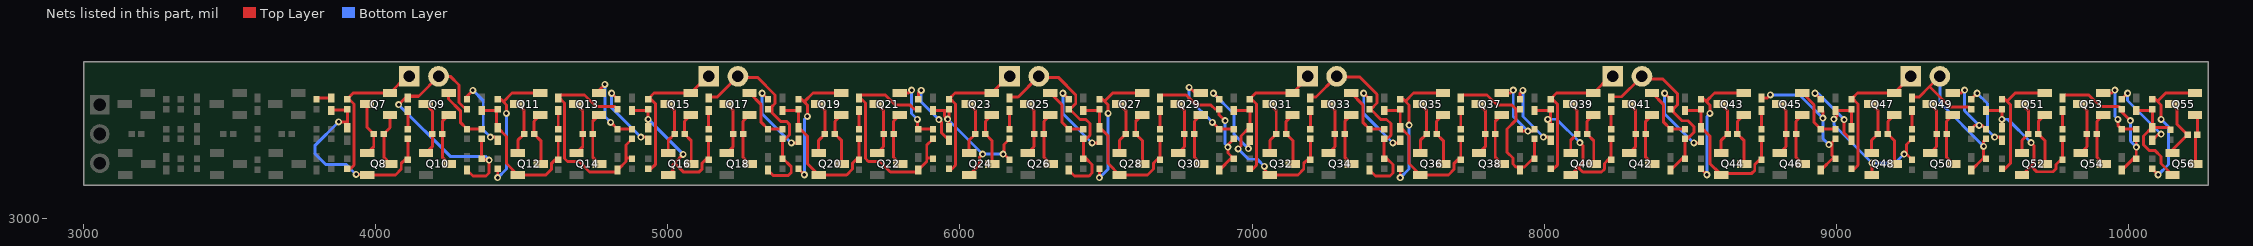
[diagram p0: the nets of this part, all layers, seen from the top]
# Altium PCB MISC51432.pcbdoc (part 2 of 2)
Units mil, origin at the board's own origin, x right, y up, seen from the top; angles counter-clockwise.
Board outline 7274.02 x 423.7 mil, 2 copper layers (Top Layer, Bottom Layer), stack 62.206 mil thick; 257 components, 141 nets, 571 pads, 133 vias.

## Via types
v1: diameter 24.02, hole 12, Top Layer to Bottom Layer, 133 vias

## Nets (pads, with @x,y where several pads share a name; then routed paths per layer and width w, separated by ;. In a path a pad name is that pad's centre, name@x,y a point inside that pad or via, vN(x,y) a via of type N, cw(c..) or ccw(c..) an arc to the next point about the centre after c; other vN are vias at no path point) (continued)
$1N4560: Q7.3 Q8.1 Rb4.2 | length 186.1
  Top Layer w10: Q7.3@3969.94,3391.14 3969.94,3311.66 Rb4.2@3992.96,3288.64 3992.96,3245.18 Q8.1@3971.32,3223.54
$1N4561: Q7.1 Q8.3 Rb4.1 | length 186.3
  Top Layer w10: Rb4.1@4027.04,3288.64 Rb4.1@4027.47,3289.07 ; Q7.1@4048.68,3353.74 4048.68,3310.28 Rb4.1@4027.47,3289.07 ; Q8.3@4050.06,3186.14 4027.47,3208.73 Rb4.1@4027.47,3289.07
$1N4562: C8.2 R6.1 | length 51.8
  Top Layer w10: R6.1@3797.5,3408.18 3801.92,3412.6 C8.2@3847.5,3412.6
$1N4850: C9.1 C10.2 H2.2 R10.2 R11.1 Rs5.2 | length 1018.2
  Top Layer w10: v1(4077.82,3388.97) 4107.82,3418.97 4147.82,3418.97 ; C9.1@4109.62,3412.6 4113.16,3416.14 4145,3416.14 4147.82,3418.97 ; C10.2@4312.5,3164.68 4332.5,3144.68 4377.82,3144.68 4387.82,3154.68 v1(4387.82,3198.97) 4377.82,3198.97 R11.1@4362.5,3214.29 ; R10.2@4312.5,3374.1 4307.04,3374.1 4285,3396.14 4285,3456.14 4255,3486.14 H2.2@4215,3486.14 4147.82,3418.97 ; R11.1@4362.5,3203.18 R11.1@4362.5,3214.29 ; Rs5.2@4362.5,3271.6 R11.1@4362.5,3214.29
  Bottom Layer w10: v1(4077.82,3388.97) 4254.6,3212.19 4374.6,3212.19 v1(4387.82,3198.97)
$1N4855: C9.2 R8.1 | length 64
  Top Layer w10: R8.1@4109.62,3305.68 C9.2@4109.62,3369.68
$1N4859: Q9.3 Q10.1 Rb5.2 | length 186.1
  Top Layer w10: Q9.3@4170.63,3391.14 4193.65,3368.12 Rb5.2@4193.65,3288.64 4193.65,3245.18 Q10.1@4172.01,3223.54
$1N4860: Q9.1 Q10.3 Rb5.1 | length 186.1
  Top Layer w10: Q9.1@4249.37,3353.74 4227.73,3332.1 Rb5.1@4227.73,3288.64 4227.73,3209.16 Q10.3@4250.75,3186.14
$1N4861: Q9.2 Rp5.2 Rs5.1 | length 199
  Top Layer w10: Q9.2@4249.37,3428.54 4249.37,3408.54 4289.37,3368.54 4289.37,3328.81 Rp5.2@4312.5,3305.68 Rs5.1@4362.5,3305.68
$1N5378: Q11.3 Q12.1 Rb6.2 | length 186.1
  Top Layer w10: Q11.3@4484.94,3391.14 4507.96,3368.12 Rb6.2@4507.96,3288.64 4486.32,3267 Q12.1@4486.32,3223.54
$1N5379: Q11.1 Q12.3 Rb6.1 | length 186.1
  Top Layer w10: Q11.1@4563.68,3353.74 4542.04,3332.1 Rb6.1@4542.04,3288.64 4565.06,3265.62 Q12.3@4565.06,3186.14
$1N5380: C12.2 R10.1 | length 252.7
  Top Layer w10: R10.1@4312.5,3408.18 4312.5,3418.18 v1(4332.5,3438.18) ; v1(4392.5,3278.18) 4406.5,3278.18 C12.2@4417.5,3267.18
  Bottom Layer w10: v1(4332.5,3438.18) 4367.86,3402.83 4367.86,3302.83 v1(4392.5,3278.18)
$1N5381: C11.1 C12.1 Q12.2 R12.2 R13.2 Rp6.1 | length 550.3
  Top Layer w10: C11.1@4362.5,3369.68 Rp6.1@4413.08,3369.68 ; Rp6.1@4417.5,3374.1 Rp6.1@4413.08,3369.68 ; R12.2@4624.62,3271.6 R13.2@4624.62,3201.14 4614.62,3201.14 4602.22,3188.74 4602.22,3168.74 4582.22,3148.74 Q12.2@4486.32,3148.74 4447.5,3187.56 4447.5,3280.1 C12.1@4417.5,3310.1 4413.08,3314.52 Rp6.1@4413.08,3369.68
$1N5390: Q11.2 Rp6.2 Rs6.1 | length 468.9
  Top Layer w10: v1(4417.5,3139.1) Rs6.1@4417.5,3169.1 ; Rp6.2@4417.5,3408.18 4427.5,3408.18 4436.89,3398.79 ; v1(4447.5,3359.1) 4447.5,3388.18 4436.89,3398.79 ; Q11.2@4563.68,3428.54 4466.65,3428.54 4436.89,3398.79
  Bottom Layer w10: v1(4417.5,3139.1) 4447.5,3169.1 v1(4447.5,3359.1)
$1N5401: C13.1 C14.2 R14.2 R15.1 Rs7.2 | length 804.1
  Top Layer w10: C13.1@4624.62,3412.6 C13.1@4626.39,3414.37 ; C14.2@4827.5,3164.68 4831.64,3168.82 C14.2@4831.64,3169.62 ; R14.2@4827.5,3374.1 4819,3382.6 4754.62,3382.6 4714.62,3422.6 4634.62,3422.6 C13.1@4626.39,3414.37 ; R15.1@4877.5,3203.18 4873.81,3206.87 4856.39,3206.87 ; Rs7.2@4877.5,3271.6 4856.39,3250.49 4856.39,3206.87 ; C13.1@4626.39,3414.37 4646.39,3394.37 4646.39,3204.37 4656.39,3194.37 4696.39,3194.37 4731.74,3159.01 4821.03,3159.01 C14.2@4831.64,3169.62 ; C14.2@4831.64,3169.62 4856.39,3194.37 4856.39,3206.87
$1N5406: C13.2 R12.1 | length 64
  Top Layer w10: R12.1@4624.62,3305.68 C13.2@4624.62,3369.68
$1N5415: Q13.3 Q14.1 Rb7.2 | length 186.1
  Top Layer w10: Q13.3@4685.63,3391.14 4708.65,3368.12 Rb7.2@4708.65,3288.64 4708.65,3245.18 Q14.1@4687.01,3223.54
$1N5416: Q13.1 Q14.3 Rb7.1 | length 186.1
  Top Layer w10: Q13.1@4764.37,3353.74 4742.73,3332.1 Rb7.1@4742.73,3288.64 4742.73,3209.16 Q14.3@4765.75,3186.14
$1N5417: Q13.2 Rp7.2 Rs7.1 | length 259.1
  Top Layer w10: Q13.2@4764.37,3428.54 4764.37,3438.54 v1(4784.37,3458.54) ; v1(4804.37,3328.54) Rp7.2@4827.5,3305.68 Rs7.1@4877.5,3305.68
  Bottom Layer w10: v1(4784.37,3458.54) 4784.37,3348.54 v1(4804.37,3328.54)
$1N5932: Q15.3 Q16.1 Rb8.2 | length 186.1
  Top Layer w10: Q15.3@4999.94,3391.14 5022.96,3368.12 Rb8.2@5022.96,3288.64 5001.32,3267 Q16.1@5001.32,3223.54
$1N5933: Q15.1 Q16.3 Rb8.1 | length 186.1
  Top Layer w10: Q15.1@5078.68,3353.74 5057.04,3332.1 Rb8.1@5057.04,3288.64 5080.06,3265.62 Q16.3@5080.06,3186.14
$1N5934: C16.2 R14.1 | length 249.3
  Top Layer w10: v1(4807.5,3428.18) R14.1@4827.5,3408.18 ; v1(4907.5,3278.18) 4921.5,3278.18 C16.2@4932.5,3267.18
  Bottom Layer w10: v1(4807.5,3428.18) 4807.5,3378.18 v1(4907.5,3278.18)
$1N5955: C17.1 C18.2 H3.2 R18.2 R19.1 Rs9.2 | length 732.3
  Top Layer w10: C17.1@5139.62,3412.6 5142.45,3415.43 5169.29,3415.43 H3.2@5236.46,3482.61 ; H3.2@5240,3486.14 H3.2@5236.46,3482.61 ; C18.2@5342.5,3164.68 5360.58,3146.6 5412.5,3146.6 5422.5,3156.6 5422.5,3176.6 R19.1@5392.5,3206.6 ; R18.2@5342.5,3374.1 5347.96,3374.1 5355.86,3382 ; R19.1@5392.5,3203.18 R19.1@5392.5,3206.6 ; H3.2@5236.46,3482.61 5306.46,3482.61 5366.46,3422.61 5366.46,3392.61 5355.86,3382 ; 5355.86,3382 5355.86,3362 5385.86,3332 5405.86,3332 5415.86,3322 5415.86,3284.96 5402.5,3271.6 Rs9.2@5392.5,3271.6 R19.1@5392.5,3206.6
$1N5960: C17.2 R16.1 | length 64
  Top Layer w10: R16.1@5139.62,3305.68 C17.2@5139.62,3369.68
$1N5969: Q17.3 Q18.1 Rb9.2 | length 186.1
  Top Layer w10: Q17.3@5200.63,3391.14 5223.65,3368.12 Rb9.2@5223.65,3288.64 5223.65,3245.18 Q18.1@5202.01,3223.54
$1N5970: Q17.1 Q18.3 Rb9.1 | length 186.1
  Top Layer w10: Q17.1@5279.37,3353.74 5257.73,3332.1 Rb9.1@5257.73,3288.64 5257.73,3209.16 Q18.3@5280.75,3186.14
$1N6486: Q19.3 Q20.1 Rb10.2 | length 186.1
  Top Layer w10: Q19.3@5514.94,3391.14 5537.96,3368.12 Rb10.2@5537.96,3288.64 5516.32,3267 Q20.1@5516.32,3223.54
$1N6487: Q19.1 Q20.3 Rb10.1 | length 186.1
  Top Layer w10: Q19.1@5593.68,3353.74 5572.04,3332.1 Rb10.1@5572.04,3288.64 5595.06,3265.62 Q20.3@5595.06,3186.14
$1N6488: C20.2 R18.1 | length 268.4
  Top Layer w10: v1(5322.5,3428.18) R18.1@5342.5,3408.18 ; v1(5422.5,3258.18) 5438.5,3258.18 C20.2@5447.5,3267.18
  Bottom Layer w10: v1(5322.5,3428.18) 5322.5,3358.18 v1(5422.5,3258.18)
$1N6489: C19.1 C20.1 Q20.2 R20.2 R21.2 Rp10.1 | length 554.4
  Top Layer w10: C19.1@5392.5,3369.68 5443.08,3369.68 Rp10.1@5447.5,3374.1 C20.1@5447.5,3311.6 ; C20.1@5447.5,3310.1 C20.1@5447.5,3311.6 ; R20.2@5654.62,3271.6 R21.2@5654.62,3201.14 5644.62,3201.14 5632.22,3188.74 5632.22,3168.74 5612.22,3148.74 Q20.2@5516.32,3148.74 5477.5,3187.56 5477.5,3281.6 C20.1@5447.5,3311.6
$1N6498: Q19.2 Rp10.2 Rs10.1 | length 448.9
  Top Layer w10: Rs10.1@5447.5,3169.1 v1(5467.5,3149.1) ; Rp10.2@5447.5,3408.18 5457.5,3408.18 5466.89,3398.79 ; v1(5477.5,3349.1) 5477.5,3388.18 5466.89,3398.79 ; Q19.2@5593.68,3428.54 5496.65,3428.54 5466.89,3398.79
  Bottom Layer w10: v1(5467.5,3149.1) 5467.5,3339.1 v1(5477.5,3349.1)
$1N6509: C21.1 C22.2 R22.2 R23.1 Rs11.2 | length 797.4
  Top Layer w10: C21.1@5654.62,3412.6 C21.1@5656.39,3414.37 ; R22.2@5857.5,3374.1 5843.12,3374.1 5829.97,3387.25 5779.97,3387.25 5744.62,3422.6 5664.62,3422.6 C21.1@5656.39,3414.37 ; R23.1@5907.5,3203.18 5903.81,3206.87 5886.39,3206.87 ; Rs11.2@5907.5,3271.6 5886.39,3250.49 5886.39,3206.87 ; C21.1@5656.39,3414.37 5676.39,3394.37 5676.39,3204.37 5686.39,3194.37 5726.39,3194.37 5761.74,3159.01 5851.03,3159.01 5886.39,3194.37 5886.39,3206.87
$1N6514: C21.2 R20.1 | length 64
  Top Layer w10: R20.1@5654.62,3305.68 C21.2@5654.62,3369.68
$1N6523: Q21.3 Q22.1 Rb11.2 | length 186.1
  Top Layer w10: Q21.3@5715.63,3391.14 5738.65,3368.12 Rb11.2@5738.65,3288.64 5738.65,3245.18 Q22.1@5717.01,3223.54
$1N6524: Q21.1 Q22.3 Rb11.1 | length 186.1
  Top Layer w10: Q21.1@5794.37,3353.74 5772.73,3332.1 Rb11.1@5772.73,3288.64 5772.73,3209.16 Q22.3@5795.75,3186.14
$1N6525: Q21.2 Rp11.2 Rs11.1 | length 236.6
  Top Layer w10: Q21.2@5794.37,3428.54 5824.37,3428.54 v1(5834.37,3438.54) ; v1(5854.37,3338.54) 5854.37,3308.81 Rp11.2@5857.5,3305.68 Rs11.1@5907.5,3305.68
  Bottom Layer w10: v1(5834.37,3438.54) 5834.37,3358.54 v1(5854.37,3338.54)
$1N7040: Q23.3 Q24.1 Rb12.2 | length 186.1
  Top Layer w10: Q23.3@6029.94,3391.14 6052.96,3368.12 Rb12.2@6052.96,3288.64 6031.32,3267 Q24.1@6031.32,3223.54
$1N7041: Q23.1 Q24.3 Rb12.1 | length 186.1
  Top Layer w10: Q23.1@6108.68,3353.74 6087.04,3332.1 Rb12.1@6087.04,3288.64 6110.06,3265.62 Q24.3@6110.06,3186.14
$1N7042: C24.2 R22.1 | length 244.5
  Top Layer w10: R22.1@5857.5,3408.18 5857.5,3428.18 v1(5867.5,3438.18) ; v1(5927.5,3338.18) 5937.5,3328.18 5937.5,3292.18 C24.2@5962.5,3267.18
  Bottom Layer w10: v1(5867.5,3438.18) 5867.5,3398.18 v1(5927.5,3338.18)
$1N7063: C25.1 C26.2 H4.2 R26.2 R27.1 Rs13.2 | length 734.5
  Top Layer w10: C25.1@6169.62,3412.6 6172.45,3415.43 6199.29,3415.43 H4.2@6266.46,3482.61 ; H4.2@6270,3486.14 H4.2@6266.46,3482.61 ; C26.2@6372.5,3164.68 6392.5,3144.68 6442.5,3144.68 6452.5,3154.68 6452.5,3184.1 6432.5,3204.1 R27.1@6422.5,3204.1 ; R26.2@6372.5,3374.1 R26.2@6375.46,3374.1 ; R27.1@6422.5,3203.18 R27.1@6422.5,3204.1 ; H4.2@6266.46,3482.61 6336.46,3482.61 6396.46,3422.61 6396.46,3392.61 6377.96,3374.1 R26.2@6375.46,3374.1 ; R26.2@6375.46,3374.1 6410.82,3338.75 6430.82,3338.75 6445.46,3324.1 6445.46,3284.56 6432.5,3271.6 Rs13.2@6422.5,3271.6 R27.1@6422.5,3204.1
$1N7068: C25.2 R24.1 | length 64
  Top Layer w10: R24.1@6169.62,3305.68 C25.2@6169.62,3369.68
$1N7077: Q25.3 Q26.1 Rb13.2 | length 186.1
  Top Layer w10: Q25.3@6230.63,3391.14 6253.65,3368.12 Rb13.2@6253.65,3288.64 6253.65,3245.18 Q26.1@6232.01,3223.54
$1N7078: Q25.1 Q26.3 Rb13.1 | length 186.1
  Top Layer w10: Q25.1@6309.37,3353.74 6287.73,3332.1 Rb13.1@6287.73,3288.64 6287.73,3209.16 Q26.3@6310.75,3186.14
$1N7594: Q27.3 Q28.1 Rb14.2 | length 186.1
  Top Layer w10: Q27.3@6544.94,3391.14 6567.96,3368.12 Rb14.2@6567.96,3288.64 6546.32,3267 Q28.1@6546.32,3223.54
$1N7595: Q27.1 Q28.3 Rb14.1 | length 186.1
  Top Layer w10: Q27.1@6623.68,3353.74 6602.04,3332.1 Rb14.1@6602.04,3288.64 6625.06,3265.62 Q28.3@6625.06,3186.14
$1N7596: C28.2 R26.1 | length 268.4
  Top Layer w10: v1(6352.5,3428.18) R26.1@6372.5,3408.18 ; v1(6452.5,3258.18) 6468.5,3258.18 C28.2@6477.5,3267.18
  Bottom Layer w10: v1(6352.5,3428.18) 6352.5,3358.18 v1(6452.5,3258.18)
$1N7597: C27.1 C28.1 Q28.2 R28.2 R29.2 Rp14.1 | length 554.4
  Top Layer w10: C27.1@6422.5,3369.68 6473.08,3369.68 Rp14.1@6477.5,3374.1 C28.1@6477.5,3311.6 ; C28.1@6477.5,3310.1 C28.1@6477.5,3311.6 ; R28.2@6684.62,3271.6 R29.2@6684.62,3201.14 6674.62,3201.14 6662.22,3188.74 6662.22,3168.74 6642.22,3148.74 Q28.2@6546.32,3148.74 6507.5,3187.56 6507.5,3281.6 C28.1@6477.5,3311.6
$1N7606: Q27.2 Rp14.2 Rs14.1 | length 469.9
  Top Layer w10: v1(6477.5,3139.1) Rs14.1@6477.5,3169.1 ; Rp14.2@6477.5,3408.18 6487.5,3408.18 6495.13,3400.55 ; v1(6507.5,3359.1) 6507.5,3388.18 6495.13,3400.55 ; Q27.2@6623.68,3428.54 6523.11,3428.54 6495.13,3400.55
  Bottom Layer w10: v1(6477.5,3139.1) 6507.5,3169.1 v1(6507.5,3359.1)
$1N7617: C29.1 C30.2 R30.2 R31.1 Rs15.2 | length 517
  Top Layer w10: C29.1@6684.62,3412.6 6694.62,3422.6 6774.62,3422.6 6809.97,3387.25 6859.97,3387.25 6873.12,3374.1 R30.2@6887.5,3374.1 6887.5,3354.1 v1(6907.5,3334.1) ; C30.2@6887.5,3164.68 R31.1@6931.64,3208.82 ; R31.1@6937.5,3203.18 6917.5,3223.18 v1(6917.5,3244.1) 6917.5,3251.6 Rs15.2@6937.5,3271.6
  Bottom Layer w10: v1(6907.5,3334.1) 6907.5,3254.1 v1(6917.5,3244.1)
$1N7622: C29.2 R28.1 | length 64
  Top Layer w10: R28.1@6684.62,3305.68 C29.2@6684.62,3369.68
$1N7631: Q29.3 Q30.1 Rb15.2 | length 186.1
  Top Layer w10: Q29.3@6745.63,3391.14 6768.65,3368.12 Rb15.2@6768.65,3288.64 6768.65,3245.18 Q30.1@6747.01,3223.54
$1N7632: Q29.1 Q30.3 Rb15.1 | length 186.1
  Top Layer w10: Q29.1@6824.37,3353.74 6802.73,3332.1 Rb15.1@6802.73,3288.64 6802.73,3209.16 Q30.3@6825.75,3186.14
$1N7633: Q29.2 Rp15.2 Rs15.1 | length 283.9
  Top Layer w10: v1(6784.37,3448.54) 6804.37,3428.54 Q29.2@6824.37,3428.54 ; v1(6864.37,3328.54) Rp15.2@6887.5,3305.68 Rs15.1@6937.5,3305.68
  Bottom Layer w10: v1(6784.37,3448.54) 6784.37,3408.54 v1(6864.37,3328.54)
$1N8148: Q31.3 Q32.1 Rb16.2 | length 186.1
  Top Layer w10: Q31.3@7059.94,3391.14 7082.96,3368.12 Rb16.2@7082.96,3288.64 7061.32,3267 Q32.1@7061.32,3223.54
$1N8149: Q31.1 Q32.3 Rb16.1 | length 186.1
  Top Layer w10: Q31.1@7138.68,3353.74 7117.04,3332.1 Rb16.1@7117.04,3288.64 7140.06,3265.62 Q32.3@7140.06,3186.14
$1N8150: C32.2 R30.1 | length 299.1
  Top Layer w10: v1(6867.5,3428.18) R30.1@6887.5,3408.18 ; v1(6987.5,3238.18) 6987.5,3262.18 C32.2@6992.5,3267.18
  Bottom Layer w10: v1(6867.5,3428.18) 6938.21,3357.47 6938.21,3287.47 v1(6987.5,3238.18)
$1N8171: C33.1 C34.2 H5.2 R34.2 R35.1 Rs17.2 | length 737
  Top Layer w10: C33.1@7199.62,3412.6 7202.45,3415.43 7219.29,3415.43 H5.2@7288.23,3484.37 ; H5.2@7290,3486.14 H5.2@7288.23,3484.37 ; C34.2@7402.5,3164.68 7422.5,3144.68 7472.5,3144.68 7482.5,3154.68 7482.5,3184.1 7462.5,3204.1 R35.1@7452.5,3204.1 ; R34.2@7402.5,3374.1 R34.2@7405.46,3374.1 ; R35.1@7452.5,3203.18 R35.1@7452.5,3204.1 ; H5.2@7288.23,3484.37 7368.23,3484.37 7428.23,3424.37 7428.23,3394.37 7407.96,3374.1 R34.2@7405.46,3374.1 ; R34.2@7405.46,3374.1 7440.82,3338.75 7460.82,3338.75 7475.46,3324.1 7475.46,3284.56 7462.5,3271.6 Rs17.2@7452.5,3271.6 R35.1@7452.5,3204.1
$1N8176: C33.2 R32.1 | length 64
  Top Layer w10: R32.1@7199.62,3305.68 C33.2@7199.62,3369.68
$1N8185: Q33.3 Q34.1 Rb17.2 | length 186.1
  Top Layer w10: Q33.3@7260.63,3391.14 7283.65,3368.12 Rb17.2@7283.65,3288.64 7283.65,3245.18 Q34.1@7262.01,3223.54
$1N8186: Q33.1 Q34.3 Rb17.1 | length 186.1
  Top Layer w10: Q33.1@7339.37,3353.74 7317.73,3332.1 Rb17.1@7317.73,3288.64 7317.73,3209.16 Q34.3@7340.75,3186.14
$1N8702: Q35.3 Q36.1 Rb18.2 | length 186.1
  Top Layer w10: Q35.3@7574.94,3391.14 7597.96,3368.12 Rb18.2@7597.96,3288.64 7576.32,3267 Q36.1@7576.32,3223.54
$1N8703: Q35.1 Q36.3 Rb18.1 | length 186.1
  Top Layer w10: Q35.1@7653.68,3353.74 7632.04,3332.1 Rb18.1@7632.04,3288.64 7655.06,3265.62 Q36.3@7655.06,3186.14
$1N8704: C36.2 R34.1 | length 268.4
  Top Layer w10: v1(7382.5,3428.18) R34.1@7402.5,3408.18 ; v1(7482.5,3258.18) 7498.5,3258.18 C36.2@7507.5,3267.18
  Bottom Layer w10: v1(7382.5,3428.18) 7382.5,3358.18 v1(7482.5,3258.18)
$1N8705: C35.1 C36.1 Q36.2 R36.2 R37.2 Rp18.1 | length 554.4
  Top Layer w10: C35.1@7452.5,3369.68 7503.08,3369.68 Rp18.1@7507.5,3374.1 C36.1@7507.5,3311.6 ; C36.1@7507.5,3310.1 C36.1@7507.5,3311.6 ; R36.2@7714.62,3271.6 R37.2@7714.62,3201.14 7704.62,3201.14 7692.22,3188.74 7692.22,3168.74 7672.22,3148.74 Q36.2@7576.32,3148.74 7537.5,3187.56 7537.5,3281.6 C36.1@7507.5,3311.6
$1N8714: Q35.2 Rp18.2 Rs18.1 | length 469.9
  Top Layer w10: v1(7507.5,3139.1) Rs18.1@7507.5,3169.1 ; Rp18.2@7507.5,3408.18 7517.5,3408.18 7525.12,3400.55 ; v1(7537.5,3319.1) 7537.5,3388.18 7525.12,3400.55 ; Q35.2@7653.68,3428.54 7553.11,3428.54 7525.12,3400.55
  Bottom Layer w10: v1(7507.5,3139.1) 7537.5,3169.1 v1(7537.5,3319.1)
$1N8725: C37.1 C38.2 R38.2 R39.1 Rs19.2 | length 609
  Top Layer w10: C37.1@7714.62,3412.6 7724.62,3422.6 7804.62,3422.6 7839.97,3387.25 7889.97,3387.25 7903.12,3374.1 ; C38.2@7917.5,3164.68 7920.62,3167.8 C38.2@7920.62,3175.98 ; R38.2@7917.5,3374.1 7903.12,3374.1 ; R39.1@7967.5,3203.18 R39.1@7966.7,3209.57 ; Rs19.2@7967.5,3271.6 7967.5,3210.36 R39.1@7966.7,3209.57 ; 7903.12,3374.1 7903.12,3335.98 7873.12,3305.98 7873.12,3225.98 7893.12,3205.98 7893.12,3185.98 7903.12,3175.98 C38.2@7920.62,3175.98 ; C38.2@7920.62,3175.98 7933.12,3175.98 R39.1@7966.7,3209.57
$1N8730: C37.2 R36.1 | length 64
  Top Layer w10: R36.1@7714.62,3305.68 C37.2@7714.62,3369.68
$1N8739: Q37.3 Q38.1 Rb19.2 | length 186.1
  Top Layer w10: Q37.3@7775.63,3391.14 7798.65,3368.12 Rb19.2@7798.65,3288.64 7798.65,3245.18 Q38.1@7777.01,3223.54
$1N8740: Q37.1 Q38.3 Rb19.1 | length 186.1
  Top Layer w10: Q37.1@7854.37,3353.74 7832.73,3332.1 Rb19.1@7832.73,3288.64 7832.73,3209.16 Q38.3@7855.75,3186.14
$1N8741: Q37.2 Rp19.2 Rs19.1 | length 260.8
  Top Layer w10: Q37.2@7854.37,3428.54 7884.37,3428.54 v1(7894.37,3438.54) ; Rp19.2@7917.5,3305.68 7924.64,3298.54 v1(7944.37,3298.54) 7960.36,3298.54 Rs19.1@7967.5,3305.68
  Bottom Layer w10: v1(7894.37,3438.54) 7894.37,3348.54 v1(7944.37,3298.54)
$1N9256: Q39.3 Q40.1 Rb20.2 | length 186.1
  Top Layer w10: Q39.3@8089.94,3391.14 8112.96,3368.12 Rb20.2@8112.96,3288.64 8091.32,3267 Q40.1@8091.32,3223.54
$1N9257: Q39.1 Q40.3 Rb20.1 | length 186.1
  Top Layer w10: Q39.1@8168.68,3353.74 8147.04,3332.1 Rb20.1@8147.04,3288.64 8170.06,3265.62 Q40.3@8170.06,3186.14
$1N9258: C40.2 R38.1 | length 252.7
  Top Layer w10: R38.1@7917.5,3408.18 7917.5,3428.18 v1(7927.5,3438.18) ; v1(7997.5,3278.18) 8011.5,3278.18 C40.2@8022.5,3267.18
  Bottom Layer w10: v1(7927.5,3438.18) 7927.5,3348.18 v1(7997.5,3278.18)
$1N9279: C41.1 C42.2 H6.2 R42.2 R43.1 Rs21.2 | length 651.2
  Top Layer w10: C41.1@8229.62,3412.6 8233.16,3416.14 8265,3416.14 H6.2@8326.16,3477.3 ; H6.2@8335,3486.14 H6.2@8326.16,3477.3 ; C42.2@8432.5,3164.68 8474.42,3206.6 R43.1@8482.5,3206.6 ; R42.2@8432.5,3374.1 R42.2@8442.5,3374.1 ; R43.1@8482.5,3203.18 R43.1@8482.5,3206.6 ; H6.2@8326.16,3477.3 8406.16,3477.3 8456.16,3427.3 8456.16,3387.76 R42.2@8442.5,3374.1 ; R42.2@8442.5,3374.1 8442.5,3364.1 8472.5,3334.1 8492.5,3334.1 8512.5,3314.1 8512.5,3294.1 8490,3271.6 Rs21.2@8482.5,3271.6 R43.1@8482.5,3206.6
$1N9284: C41.2 R40.1 | length 64
  Top Layer w10: R40.1@8229.62,3305.68 C41.2@8229.62,3369.68
$1N9293: Q41.3 Q42.1 Rb21.2 | length 186.1
  Top Layer w10: Q41.3@8290.63,3391.14 8313.65,3368.12 Rb21.2@8313.65,3288.64 8313.65,3245.18 Q42.1@8292.01,3223.54
$1N9294: Q41.1 Q42.3 Rb21.1 | length 186.1
  Top Layer w10: Q41.1@8369.37,3353.74 8347.73,3332.1 Rb21.1@8347.73,3288.64 8347.73,3209.16 Q42.3@8370.75,3186.14
$1N9810: Q43.3 Q44.1 Rb22.2 | length 186.1
  Top Layer w10: Q43.3@8604.94,3391.14 8627.96,3368.12 Rb22.2@8627.96,3288.64 8606.32,3267 Q44.1@8606.32,3223.54
$1N9811: Q43.1 Q44.3 Rb22.1 | length 186.1
  Top Layer w10: Q43.1@8683.68,3353.74 8662.04,3332.1 Rb22.1@8662.04,3288.64 8685.06,3265.62 Q44.3@8685.06,3186.14
$1N9812: C44.2 R42.1 | length 268.4
  Top Layer w10: v1(8412.5,3428.18) R42.1@8432.5,3408.18 ; v1(8512.5,3258.18) 8528.5,3258.18 C44.2@8537.5,3267.18
  Bottom Layer w10: v1(8412.5,3428.18) 8412.5,3358.18 v1(8512.5,3258.18)
$1N9813: C43.1 C44.1 Q44.2 R44.2 R45.2 Rp22.1 | length 557.4
  Top Layer w10: C43.1@8482.5,3369.68 8533.08,3369.68 Rp22.1@8537.5,3374.1 C44.1@8537.5,3311.6 ; C44.1@8537.5,3310.1 C44.1@8537.5,3311.6 ; Q44.2@8606.32,3148.74 Q44.2@8601.09,3153.97 ; R44.2@8744.62,3271.6 R45.2@8744.62,3201.14 8738.25,3201.14 8721.09,3183.97 8721.09,3163.97 8711.09,3153.97 Q44.2@8601.09,3153.97 ; C44.1@8537.5,3311.6 8567.5,3281.6 8567.5,3187.56 Q44.2@8601.09,3153.97
$1N9822: Q43.2 Rp22.2 Rs22.1 | length 449.9
  Top Layer w10: Rs22.1@8537.5,3169.1 v1(8557.5,3149.1) ; Rp22.2@8537.5,3408.18 8547.5,3408.18 8555.12,3400.55 ; v1(8567.5,3359.1) 8567.5,3388.18 8555.12,3400.55 ; Q43.2@8683.68,3428.54 8583.11,3428.54 8555.12,3400.55
  Bottom Layer w10: v1(8557.5,3149.1) 8557.5,3349.1 v1(8567.5,3359.1)
$1N9833: C45.1 C46.2 R46.2 R47.1 Rs23.2 | length 535.3
  Top Layer w10: C45.1@8744.62,3412.6 8764.62,3412.6 v1(8774.62,3422.6) ; C46.2@8947.5,3164.68 8990.86,3208.04 R47.1@8992.64,3208.04 ; R46.2@8947.5,3374.1 8954.62,3366.98 v1(8954.62,3342.6) ; v1(8974.62,3252.6) 8978.5,3252.6 8985.57,3259.67 ; R47.1@8997.5,3203.18 R47.1@8992.64,3208.04 ; Rs23.2@8997.5,3271.6 8985.57,3259.67 ; 8985.57,3259.67 8985.57,3215.11 R47.1@8992.64,3208.04
  Bottom Layer w10: v1(8774.62,3422.6) 8874.62,3422.6 v1(8954.62,3342.6) 8954.62,3272.6 v1(8974.62,3252.6)
$1N9838: C45.2 R44.1 | length 64
  Top Layer w10: R44.1@8744.62,3305.68 C45.2@8744.62,3369.68
$1N9847: Q45.3 Q46.1 Rb23.2 | length 186.1
  Top Layer w10: Q45.3@8805.63,3391.14 8828.65,3368.12 Rb23.2@8828.65,3288.64 8828.65,3245.18 Q46.1@8807.01,3223.54
$1N9848: Q45.1 Q46.3 Rb23.1 | length 186.1
  Top Layer w10: Q45.1@8884.37,3353.74 8862.73,3332.1 Rb23.1@8862.73,3288.64 8862.73,3209.16 Q46.3@8885.75,3186.14
$1N9849: Q45.2 Rp23.2 Rs23.1 | length 199
  Top Layer w10: Q45.2@8884.37,3428.54 8924.37,3388.54 8924.37,3328.81 Rp23.2@8947.5,3305.68 Rs23.1@8997.5,3305.68
$1N10364: Q47.3 Q48.1 Rb24.2 | length 186.1
  Top Layer w10: Q47.3@9119.94,3391.14 9142.96,3368.12 Rb24.2@9142.96,3288.64 9121.32,3267 Q48.1@9121.32,3223.54
$1N10365: Q47.1 Q48.3 Rb24.1 | length 186.1
  Top Layer w10: Q47.1@9198.68,3353.74 9177.04,3332.1 Rb24.1@9177.04,3288.64 9200.06,3265.62 Q48.3@9200.06,3186.14
$1N10366: C48.2 R46.1 | length 246.9
  Top Layer w10: v1(8927.5,3428.18) R46.1@8947.5,3408.18 ; v1(9027.5,3338.18) 9027.5,3292.18 C48.2@9052.5,3267.18
  Bottom Layer w10: v1(8927.5,3428.18) 8937.5,3428.18 v1(9027.5,3338.18)
$1N10387: C49.1 C50.2 H7.2 R50.2 R51.1 Rs25.2 | length 743.2
  Top Layer w10: C49.1@9259.62,3412.6 9262.45,3415.43 9284.29,3415.43 9319.64,3450.79 ; H7.2@9355,3486.14 9319.64,3450.79 ; C50.2@9462.5,3164.68 9501,3203.18 R51.1@9512.5,3203.18 9505,3210.68 v1(9505,3246.14) 9505,3264.1 Rs25.2@9512.5,3271.6 ; R50.2@9462.5,3374.1 9455.81,3380.79 9389.64,3380.79 9319.64,3450.79
  Bottom Layer w10: H7.2@9355,3486.14 9355,3396.14 v1(9505,3246.14)
$1N10392: C49.2 R48.1 | length 64
  Top Layer w10: R48.1@9259.62,3305.68 C49.2@9259.62,3369.68
$1N10401: Q49.3 Q50.1 Rb25.2 | length 186.1
  Top Layer w10: Q49.3@9320.63,3391.14 9343.65,3368.12 Rb25.2@9343.65,3288.64 9343.65,3245.18 Q50.1@9322.01,3223.54
$1N10402: Q49.1 Q50.3 Rb25.1 | length 186.1
  Top Layer w10: Q49.1@9399.37,3353.74 9377.73,3332.1 Rb25.1@9377.73,3288.64 9377.73,3209.16 Q50.3@9400.75,3186.14
$1N10918: Q51.3 Q52.1 Rb26.2 | length 186.1
  Top Layer w10: Q51.3@9634.94,3391.14 9657.96,3368.12 Rb26.2@9657.96,3288.64 9636.32,3267 Q52.1@9636.32,3223.54
$1N10919: Q51.1 Q52.3 Rb26.1 | length 186.1
  Top Layer w10: Q51.1@9713.68,3353.74 9692.04,3332.1 Rb26.1@9692.04,3288.64 9715.06,3265.62 Q52.3@9715.06,3186.14
$1N10920: C52.2 R50.1 | length 232.7
  Top Layer w10: R50.1@9462.5,3408.18 v1(9482.5,3428.18) ; v1(9542.5,3278.18) 9556.5,3278.18 C52.2@9567.5,3267.18
  Bottom Layer w10: v1(9482.5,3428.18) 9517.85,3392.83 9517.85,3302.83 v1(9542.5,3278.18)
$1N10921: C51.1 C52.1 Q52.2 R52.2 R53.2 Rp26.1 | length 598.1
  Top Layer w10: C51.1@9512.5,3369.68 9563.08,3369.68 Rp26.1@9567.5,3374.1 v1(9567.5,3339.1) C52.1@9567.5,3310.1 ; Q52.2@9636.32,3148.74 9666.89,3179.31 ; v1(9667.5,3259.1) 9677.5,3249.1 9677.5,3189.92 9666.89,3179.31 ; R52.2@9774.62,3271.6 R53.2@9774.62,3201.14 9769.62,3201.14 9752.79,3184.31 9752.79,3169.31 9742.79,3159.31 9686.89,3159.31 9666.89,3179.31
  Bottom Layer w10: v1(9567.5,3339.1) 9587.5,3339.1 v1(9667.5,3259.1)
$1N10930: Q51.2 Rp26.2 Rs26.1 | length 415.8
  Top Layer w10: Rs26.1@9567.5,3169.1 9577.5,3169.1 9597.5,3189.1 9597.5,3388.18 9585.12,3400.55 ; Rp26.2@9567.5,3408.18 9577.5,3408.18 9585.12,3400.55 ; Q51.2@9713.68,3428.54 9613.11,3428.54 9585.12,3400.55
$1N10941: C53.1 C54.2 R54.2 R55.1 Rs27.2 | length 512.6
  Top Layer w10: C53.1@9774.62,3412.6 9784.62,3422.6 9864.62,3422.6 9904.62,3382.6 9969,3382.6 R54.2@9977.5,3374.1 9977.5,3364.1 v1(10007.5,3334.1) ; C54.2@9977.5,3164.68 10016.92,3204.1 R55.1@10027.5,3204.1 ; R55.1@10027.5,3203.18 R55.1@10027.5,3204.1 ; Rs27.2@10027.5,3271.6 v1(10027.5,3244.1) R55.1@10027.5,3204.1
  Bottom Layer w10: v1(10007.5,3334.1) 10007.5,3264.1 v1(10027.5,3244.1)
$1N10946: C53.2 R52.1 | length 64
  Top Layer w10: R52.1@9774.62,3305.68 C53.2@9774.62,3369.68
$1N10955: Q53.3 Q54.1 Rb27.2 | length 186.1
  Top Layer w10: Q53.3@9835.63,3391.14 9858.65,3368.12 Rb27.2@9858.65,3288.64 9858.65,3245.18 Q54.1@9837.01,3223.54
$1N10956: Q53.1 Q54.3 Rb27.1 | length 186.1
  Top Layer w10: Q53.1@9914.37,3353.74 9892.73,3332.1 Rb27.1@9892.73,3288.64 9892.73,3209.16 Q54.3@9915.75,3186.14
$1N10957: Q53.2 Rp27.2 Rs27.1 | length 236.6
  Top Layer w10: Q53.2@9914.37,3428.54 9944.37,3428.54 v1(9954.37,3438.54) ; v1(9964.37,3338.54) 9964.37,3318.81 Rp27.2@9977.5,3305.68 Rs27.1@10027.5,3305.68
  Bottom Layer w10: v1(9954.37,3438.54) 9954.37,3348.54 v1(9964.37,3338.54)
$1N11472: Q55.3 Q56.1 Rb28.2 | length 211
  Top Layer w10: Q55.3@10149.94,3391.14 10167.6,3373.47 10167.6,3321.5 Rb28.2@10202.96,3286.14 10151.32,3234.5 Q56.1@10151.32,3223.54
$1N11473: Q55.1 Q56.3 Rb28.1 | length 174
  Top Layer w10: Q55.1@10228.68,3353.74 10237.04,3345.38 Rb28.1@10237.04,3286.14 10230.06,3279.16 Q56.3@10230.06,3186.14
$1N11474: C56.2 R54.1 | length 254.6
  Top Layer w10: R54.1@9977.5,3408.18 v1(9997.5,3428.18) ; C56.2@10082.5,3267.18 10103.5,3288.18 v1(10112.5,3288.18)
  Bottom Layer w10: v1(9997.5,3428.18) 9997.5,3403.18 v1(10112.5,3288.18)
$1N11475: C55.1 C56.1 Q56.2 R56.2 Rp28.1 | length 414.8
  Top Layer w10: C55.1@10027.5,3369.68 10078.08,3369.68 Rp28.1@10082.5,3374.1 C56.1@10082.5,3311.6 ; C56.1@10082.5,3310.1 C56.1@10082.5,3311.6 ; R56.2@10145,3303.18 10136.58,3311.6 C56.1@10082.5,3311.6 ; Q56.2@10151.32,3148.74 10112.5,3187.56 10112.5,3211.6 10092.5,3231.6 10072.5,3231.6 10052.5,3251.6 10052.5,3281.6 C56.1@10082.5,3311.6
$1N11484: Q55.2 Rp28.2 Rs28.1 | length 470.9
  Top Layer w10: Rs28.1@10082.5,3169.1 v1(10102.5,3149.1) ; Rp28.2@10082.5,3408.18 10092.5,3408.18 10100.12,3400.55 ; v1(10112.5,3339.1) 10112.5,3388.18 10100.12,3400.55 ; Q55.2@10228.68,3428.54 10128.11,3428.54 10100.12,3400.55
  Bottom Layer w10: v1(10102.5,3149.1) 10137.85,3184.46 10137.85,3313.75 v1(10112.5,3339.1)
$1N12299: H2.1 Q7.2 Rp4.2 Rs4.1 | length 510.1
  Top Layer w10: Rs4.1@3902.5,3169.1 3912.5,3169.1 3925.18,3181.78 3925.18,3390.86 Rp4.2@3905.18,3410.86 ; Rp4.2@3902.5,3408.18 Rp4.2@3905.18,3410.86 ; H2.1@4115,3486.14 4106.28,3486.14 Q7.2@4048.68,3428.54 3922.86,3428.54 Rp4.2@3905.18,3410.86
$1N12309: C7.1 C8.1 Q8.2 R8.2 R9.2 Rp4.1 | length 742.9
  Top Layer w10: C8.1@3847.5,3369.68 3847.92,3370.1 Rp4.1@3902.5,3370.1 ; v1(3872.5,3330.1) 3902.5,3330.1 ; C7.1@3902.5,3310.1 3902.5,3330.1 ; Rp4.1@3902.5,3374.1 Rp4.1@3902.5,3370.1 ; v1(3932.5,3150.1) 3969.96,3150.1 Q8.2@3971.32,3148.74 4067.22,3148.74 4087.22,3168.74 4087.22,3188.74 4099.62,3201.14 R9.2@4109.62,3201.14 R8.2@4109.62,3271.6 ; 3902.5,3330.1 Rp4.1@3902.5,3370.1
  Bottom Layer w10: v1(3872.5,3330.1) 3792.5,3250.1 3792.5,3220.1 3827.86,3184.75 3897.86,3184.75 v1(3932.5,3150.1)
$1N12317: H3.1 Q15.2 Rp8.2 Rs8.1 | length 507.6
  Top Layer w10: Rs8.1@4932.5,3169.1 4942.5,3169.1 4956.95,3183.55 4956.95,3392.63 Rp8.2@4936.95,3412.63 ; Rp8.2@4932.5,3408.18 Rp8.2@4936.95,3412.63 ; H3.1@5140,3486.14 5136.28,3486.14 Q15.2@5078.68,3428.54 4952.86,3428.54 Rp8.2@4936.95,3412.63
$1N12327: C15.1 C16.1 Q16.2 R16.2 R17.2 Rp8.1 | length 611.3
  Top Layer w10: C15.1@4877.5,3369.68 4928.08,3369.68 Rp8.1@4932.5,3374.1 v1(4932.5,3339.1) C16.1@4932.5,3310.1 ; Q16.2@5001.32,3148.74 5017.14,3164.57 5017.14,3183.75 5022.45,3189.05 ; v1(5052.5,3219.1) 5022.45,3189.05 ; R16.2@5139.62,3271.6 R17.2@5139.62,3201.14 5129.62,3201.14 5117.53,3189.05 5117.53,3169.05 5107.53,3159.05 5052.45,3159.05 5022.45,3189.05
  Bottom Layer w10: v1(4932.5,3339.1) v1(5052.5,3219.1)
$1N12335: H4.1 Q23.2 Rp12.2 Rs12.1 | length 505.1
  Top Layer w10: Rs12.1@5962.5,3169.1 5972.5,3169.1 5985.18,3181.78 5985.18,3390.86 Rp12.2@5965.18,3410.86 ; Rp12.2@5962.5,3408.18 Rp12.2@5965.18,3410.86 ; H4.1@6170,3486.14 6166.28,3486.14 Q23.2@6108.68,3428.54 5982.86,3428.54 Rp12.2@5965.18,3410.86
$1N12345: C23.1 C24.1 Q24.2 R24.2 R25.2 Rp12.1 | length 574.1
  Top Layer w10: C23.1@5907.5,3369.68 5947.5,3369.68 ; v1(5957.5,3339.68) 5947.5,3349.68 5947.5,3369.68 ; C24.1@5962.5,3310.1 Rp12.1@5962.5,3374.1 5958.08,3369.68 5947.5,3369.68 ; Q24.2@6031.32,3148.74 6067.5,3184.92 6067.5,3209.68 v1(6077.5,3219.68) ; v1(6147.5,3219.68) v1@6151.08,3219.68 ; R25.2@6169.62,3201.14 v1@6151.08,3219.68 ; R24.2@6169.62,3271.6 6151.08,3253.06 v1@6151.08,3219.68
  Bottom Layer w10: v1(5957.5,3339.68) v1(6077.5,3219.68) v1(6147.5,3219.68)
$1N12353: H5.1 Q31.2 Rp16.2 Rs16.1 | length 498.8
  Top Layer w10: Rs16.1@6992.5,3169.1 7002.5,3169.1 7015.18,3181.78 7015.18,3390.86 Rp16.2@6995.18,3410.86 ; Rp16.2@6992.5,3408.18 Rp16.2@6995.18,3410.86 ; H5.1@7190,3486.14 7190,3479.86 Q31.2@7138.68,3428.54 7012.86,3428.54 Rp16.2@6995.18,3410.86
$1N12363: C31.1 C32.1 Q32.2 R32.2 R33.2 Rp16.1 | length 605.1
  Top Layer w10: C31.1@6937.5,3369.68 6988.08,3369.68 Rp16.1@6992.5,3374.1 C32.1@6992.5,3311.6 ; v1(6952.5,3237.56) 6962.5,3247.56 6962.5,3281.6 C32.1@6992.5,3311.6 ; C32.1@6992.5,3310.1 C32.1@6992.5,3311.6 ; v1(7042.5,3177.56) 7042.5,3167.56 Q32.2@7061.32,3148.74 7157.22,3148.74 7177.22,3168.74 7177.22,3188.74 7189.62,3201.14 R33.2@7199.62,3201.14 R32.2@7199.62,3271.6
  Bottom Layer w10: v1(6952.5,3237.56) 6987.85,3202.21 7017.85,3202.21 v1(7042.5,3177.56)
$1N12371: H6.1 Q39.2 Rp20.2 Rs20.1 | length 510.1
  Top Layer w10: Rs20.1@8022.5,3169.1 8032.5,3169.1 8045.18,3181.78 8045.18,3390.86 Rp20.2@8025.18,3410.86 ; Rp20.2@8022.5,3408.18 Rp20.2@8025.18,3410.86 ; H6.1@8235,3486.14 8226.28,3486.14 Q39.2@8168.68,3428.54 8042.86,3428.54 Rp20.2@8025.18,3410.86
$1N12381: C39.1 C40.1 Q40.2 R40.2 R41.2 Rp20.1 | length 625.1
  Top Layer w10: C39.1@7967.5,3369.68 8018.08,3369.68 Rp20.1@8022.5,3374.1 v1@8022.5,3339.1 ; v1(8012.5,3339.1) v1@8022.5,3339.1 ; C40.1@8022.5,3310.1 v1@8022.5,3339.1 ; Q40.2@8091.32,3148.74 8116.59,3174.01 ; v1(8122.5,3259.1) 8132.5,3249.1 8132.5,3189.92 8116.59,3174.01 ; R40.2@8229.62,3271.6 R41.2@8229.62,3201.14 8219.62,3201.14 8206.59,3188.11 8206.59,3168.11 8196.59,3158.11 8132.49,3158.11 8116.59,3174.01
  Bottom Layer w10: v1(8012.5,3339.1) 8042.5,3339.1 v1(8122.5,3259.1)
$1N12389: H7.1 Q47.2 Rp24.2 Rs24.1 | length 500.8
  Top Layer w10: Rs24.1@9052.5,3169.1 9062.5,3169.1 9075.18,3181.78 9075.18,3390.86 Rp24.2@9055.18,3410.86 ; Rp24.2@9052.5,3408.18 Rp24.2@9055.18,3410.86 ; H7.1@9255,3486.14 9255,3484.86 Q47.2@9198.68,3428.54 9072.86,3428.54 Rp24.2@9055.18,3410.86
$1N12399: C47.1 C48.1 Q48.2 R48.2 R49.2 Rp24.1 | length 617.1
  Top Layer w10: v1(8992.5,3339.68) 9002.5,3349.68 C47.1@9002.5,3369.68 ; C47.1@8997.5,3369.68 C47.1@9002.5,3369.68 ; C48.1@9052.5,3310.1 Rp24.1@9052.5,3374.1 9048.08,3369.68 C47.1@9002.5,3369.68 ; Q48.2@9121.32,3148.74 9122.5,3149.92 v1(9122.5,3189.68) ; v1(9232.5,3219.68) v1@9241.08,3219.68 ; R49.2@9259.62,3201.14 v1@9241.08,3219.68 ; R48.2@9259.62,3271.6 9241.08,3253.06 v1@9241.08,3219.68
  Bottom Layer w10: v1(8992.5,3339.68) 8992.5,3319.68 v1(9122.5,3189.68) 9202.5,3189.68 v1(9232.5,3219.68)
$1N12408: Q17.2 Rp9.2 Rs9.1 | length 199
  Top Layer w10: Q17.2@5279.37,3428.54 5319.37,3388.54 5319.37,3328.81 Rp9.2@5342.5,3305.68 Rs9.1@5392.5,3305.68
$1N12432: Q25.2 Rp13.2 Rs13.1 | length 199
  Top Layer w10: Q25.2@6309.37,3428.54 6349.37,3388.54 6349.37,3328.81 Rp13.2@6372.5,3305.68 Rs13.1@6422.5,3305.68
$1N12456: Q33.2 Rp17.2 Rs17.1 | length 199
  Top Layer w10: Q33.2@7339.37,3428.54 7379.37,3388.54 7379.37,3328.81 Rp17.2@7402.5,3305.68 Rs17.1@7452.5,3305.68
$1N12480: Q41.2 Rp21.2 Rs21.1 | length 199
  Top Layer w10: Q41.2@8369.37,3428.54 8409.37,3388.54 8409.37,3328.81 Rp21.2@8432.5,3305.68 Rs21.1@8482.5,3305.68
$1N12504: Q49.2 Rp25.2 Rs25.1 | length 245.5
  Top Layer w10: Q49.2@9399.37,3428.54 9429.37,3428.54 v1(9439.37,3438.54) ; Rp25.2@9462.5,3305.68 9475.36,3318.54 v1(9489.37,3318.54) 9499.64,3318.54 Rs25.1@9512.5,3305.68
  Bottom Layer w10: v1(9439.37,3438.54) 9439.37,3368.54 v1(9489.37,3318.54)

## Keep-outs
Board Outline Layer:
  the board outline again, w10

## Other copper
Top Layer:
  drawing of 832 lines, arcs and shapes, not listed
Bottom Layer:
  drawing of 167 lines, arcs and shapes, not listed

## Silkscreen, mask and mechanical layers (free items; w line width, h text height)
Bottom Silkscreen Layer:
  text "B1" at 4280,3341.14 h120
  text "B2" at 5305,3341.14 h120
  text "B3" at 6335,3341.14 h120
  text "B4" at 7355,3341.14 h120
  text "B5" at 8400,3341.14 h120
  text "B6" at 9420,3339.86 h120
  text "V1" at 4150,3336.14 h120
  text "V2" at 5175,3336.14 h120
  text "V3" at 6205,3336.14 h120
  text "V4" at 7225,3336.14 h120
  text "V5" at 8270,3336.14 h120
  text "V6" at 9290,3334.86 h120
  text "GND" at 3329.37,3325.82 h120
  text "B0" at 3329.37,3222.91 h120
  text "GND" at 3329.37,3120 h120